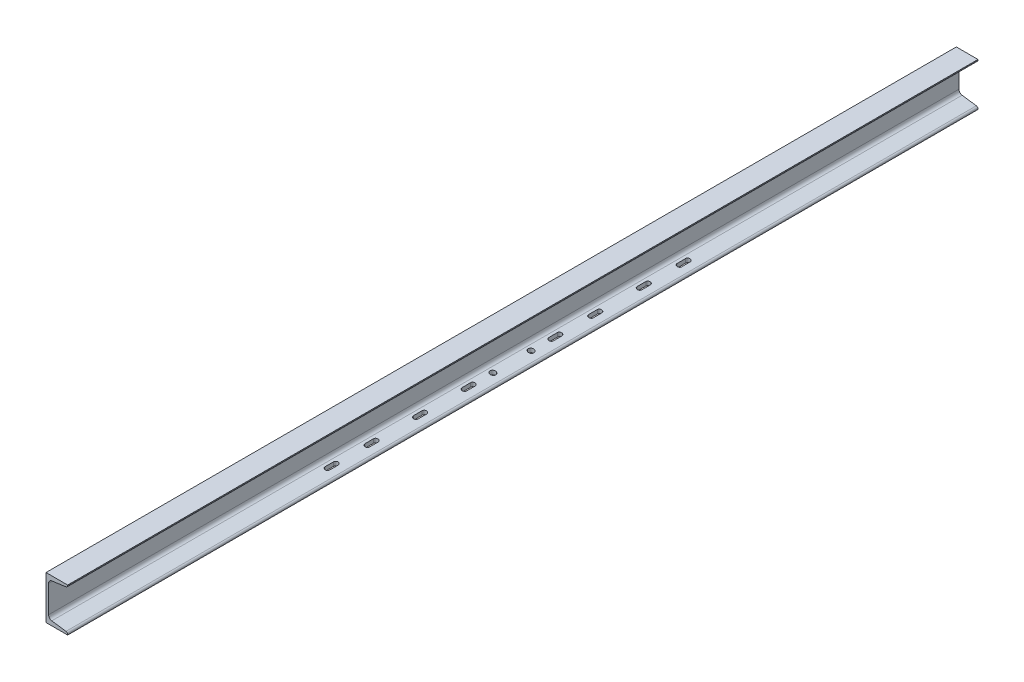
SolidWorks part; units mm, degrees
ref_plane "前视基准面" through (0, 0, 0) normal (0, 0, 1) x (1, 0, 0)
ref_plane "上视基准面" through (0, 0, 0) normal (0, 1, 0) x (1, 0, 0)
ref_plane "右视基准面" through (0, 0, 0) normal (1, 0, 0) x (0, 0, -1)
sketch "草图1" plane through (0, 0, 0) normal (0, 0, 1) x (1, 0, 0)
  line L0 (0, 0) -> (-50, 0)
  line L1 (-50, 0) -> (-50, -100)
  line L2 (-50, -100) -> (0, -100)
  line L3 (0, -100) -> (0, -98.9253)
  line L4 (-3.8737, -94.4691) -> (-36.683, -89.8581)
  line L5 (-44, -81.4408) -> (-44, -18.5592)
  line L6 (-36.683, -10.1419) -> (-3.8737, -5.5309)
  line L7 (0, -1.0747) -> (0, 0)
  line L8 (-25, -91.5) -> (-25, -100) construction
  arc A0 (-36.683, -89.8581) -> (-44, -81.4408) centre (-35.5, -81.4408) cw
  arc A1 (-44, -18.5592) -> (-36.683, -10.1419) centre (-35.5, -18.5592) cw
  arc A2 (0, -98.9253) -> (-3.8737, -94.4691) centre (-4.5, -98.9253) ccw
  arc A3 (-3.8737, -5.5309) -> (0, -1.0747) centre (-4.5, -1.0747) ccw
  dimension "D8" = 8.5
  dimension "D9" = 4.5
  dimension "D1" = 100
  dimension "D2" = 50
  dimension "D3" = 6
  dimension "D4" = 25
  dimension "D5" = 8.5
  dimension "D6" = 8
  dimension "D7" = 8
extrude "凸台-拉伸1" add sketch "草图1" along normal blind 2100
sketch "草图2" plane through (-50, 0, 0) normal (-1, 0, 0) x (0, 0, 1)
  line L0 (0, 0) -> (0, -100) construction
  line L1 (2100, 0) -> (0, 0) construction
  circle A0 centre (59.6, -30) radius 6.5
  circle A1 centre (183.4, -30) radius 6.5
  circle A2 centre (307.2, -30) radius 6.5
  circle A3 centre (431, -30) radius 6.5
  circle A4 centre (554.8, -30) radius 6.5
  circle A5 centre (678.6, -30) radius 6.5
  circle A6 centre (802.4, -30) radius 6.5
  circle A7 centre (926.2, -30) radius 6.5
  circle A8 centre (1050, -30) radius 6.5
  circle A9 centre (1173.8, -30) radius 6.5
  circle A10 centre (1297.6, -30) radius 6.5
  circle A11 centre (1421.4, -30) radius 6.5
  circle A12 centre (1545.2, -30) radius 6.5
  circle A13 centre (1669, -30) radius 6.5
  circle A14 centre (1792.8, -30) radius 6.5
  circle A15 centre (1916.6, -30) radius 6.5
  circle A16 centre (2040.4, -30) radius 6.5
  dimension "D3" = 13
  dimension "D4" = 30
  dimension "D2" = 59.6
  dimension "D1" = 17
extrude "切除-拉伸1" cut sketch "草图2" against normal blind 2100
sketch "草图6" plane through (0, -100, 0) normal (0, -1, 0) x (1, 0, 0)
  line L0 (-25, 644) -> (-25, 664) construction
  line L1 (-30.25, 644) -> (-30.25, 664)
  line L2 (-19.75, 644) -> (-19.75, 664)
  line L3 (-25, 736) -> (-25, 756) construction
  line L4 (-30.25, 736) -> (-30.25, 756)
  line L5 (-19.75, 736) -> (-19.75, 756)
  line L6 (-25, 868) -> (-25, 848) construction
  line L7 (-19.75, 868) -> (-19.75, 848)
  line L8 (-30.25, 868) -> (-30.25, 848)
  line L9 (-25, 960) -> (-25, 940) construction
  line L10 (-19.75, 960) -> (-19.75, 940)
  line L11 (-30.25, 960) -> (-30.25, 940)
  line L12 (-25, 1272) -> (-25, 1252) construction
  line L13 (-19.75, 1272) -> (-19.75, 1252)
  line L14 (-30.25, 1272) -> (-30.25, 1252)
  line L15 (-25, 1476) -> (-25, 1456) construction
  line L16 (-19.75, 1476) -> (-19.75, 1456)
  line L17 (-30.25, 1476) -> (-30.25, 1456)
  line L18 (-25, 1384) -> (-25, 1364) construction
  line L19 (-19.75, 1384) -> (-19.75, 1364)
  line L20 (-30.25, 1384) -> (-30.25, 1364)
  line L21 (-25, 1160) -> (-25, 1140) construction
  line L22 (-19.75, 1160) -> (-19.75, 1140)
  line L23 (-30.25, 1160) -> (-30.25, 1140)
  line L24 (-50, 2100) -> (-50, 0) construction
  line L26 (0, 2100) -> (0, 0) construction
  arc A0 (-30.25, 644) -> (-19.75, 644) centre (-25, 644) ccw
  arc A1 (-19.75, 664) -> (-30.25, 664) centre (-25, 664) ccw
  arc A2 (-30.25, 736) -> (-19.75, 736) centre (-25, 736) ccw
  arc A3 (-19.75, 756) -> (-30.25, 756) centre (-25, 756) ccw
  arc A4 (-19.75, 868) -> (-30.25, 868) centre (-25, 868) ccw
  arc A5 (-30.25, 848) -> (-19.75, 848) centre (-25, 848) ccw
  arc A6 (-19.75, 960) -> (-30.25, 960) centre (-25, 960) ccw
  arc A7 (-30.25, 940) -> (-19.75, 940) centre (-25, 940) ccw
  arc A8 (-19.75, 1272) -> (-30.25, 1272) centre (-25, 1272) ccw
  arc A9 (-30.25, 1252) -> (-19.75, 1252) centre (-25, 1252) ccw
  arc A10 (-19.75, 1476) -> (-30.25, 1476) centre (-25, 1476) ccw
  arc A11 (-30.25, 1456) -> (-19.75, 1456) centre (-25, 1456) ccw
  arc A12 (-19.75, 1384) -> (-30.25, 1384) centre (-25, 1384) ccw
  arc A13 (-30.25, 1364) -> (-19.75, 1364) centre (-25, 1364) ccw
  arc A14 (-19.75, 1160) -> (-30.25, 1160) centre (-25, 1160) ccw
  arc A15 (-30.25, 1140) -> (-19.75, 1140) centre (-25, 1140) ccw
  circle A16 centre (-25, 1006) radius 6.5
  circle A17 centre (-25, 1094) radius 6.5
  point P2 (-25, 654)
  point P7 (-25, 746)
  point P16 (-25, 858)
  point P21 (-25, 950)
  point P28 (-25, 1262)
  point P35 (-25, 1466)
  point P42 (-25, 1374)
  point P49 (-25, 1150)
  point P58 (-50, 1050)
  point P65 (0, 0)
  dimension "D12" = 13
  dimension "D13" = 13
  dimension "D1" = 92
  dimension "D2" = 10.5
  dimension "D3" = 20
  dimension "D4" = 112
  dimension "D5" = 92
  dimension "D6" = 200
  dimension "D7" = 100
  dimension "D8" = 112
  dimension "D9" = 92
  dimension "D10" = 112
  dimension "D11" = 25
  dimension "D14" = 88
  dimension "D15" = 44
extrude "切除-拉伸3" cut sketch "草图6" against normal blind 10
